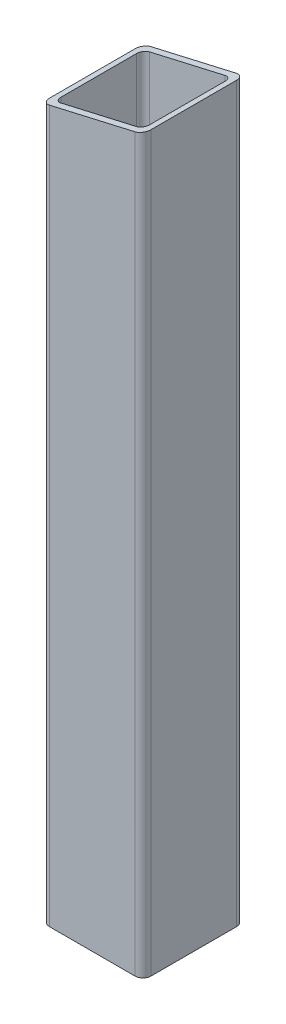
from build123d import *

# Parameters (mm, degrees)
BOSS_EXTRUDE1_DEPTH = 361.5
CUT_EXTRUDE1_REACH  = 390.178


with BuildPart() as part:
    # Sketch2 → Boss-Extrude1 (new, symmetric)
    with BuildSketch(Plane(origin=(0, 0, 0), x_dir=(1, 0, 0), z_dir=(0, 1, 0))):
        with BuildLine():
            Line((7.875, -1.525), (92.125, -1.525))
            ThreePointArc((92.125, -1.525), (97.693465902, 0.781534098), (100, 6.35))
            Line((100, 6.35), (100, 90.6))
            ThreePointArc((100, 90.6), (97.693465902, 96.168465902), (92.125, 98.475))
            Line((92.125, 98.475), (7.875, 98.475))
            ThreePointArc((7.875, 98.475), (2.306534098, 96.168465902), (0, 90.6))
            Line((0, 90.6), (0, 6.35))
            ThreePointArc((0, 6.35), (2.306534098, 0.781534098), (7.875, -1.525))
        make_face()
        with BuildLine():
            Line((12.6, 4.775), (87.4, 4.775))
            ThreePointArc((87.4, 4.775), (91.854772721, 6.620227279), (93.7, 11.075))
            Line((93.7, 11.075), (93.7, 85.875))
            ThreePointArc((93.7, 85.875), (91.854772721, 90.329772721), (87.4, 92.175))
            Line((87.4, 92.175), (12.6, 92.175))
            ThreePointArc((12.6, 92.175), (8.145227279, 90.329772721), (6.3, 85.875))
            Line((6.3, 85.875), (6.3, 11.075))
            ThreePointArc((6.3, 11.075), (8.145227279, 6.620227279), (12.6, 4.775))
        make_face(mode=Mode.SUBTRACT)
    extrude(amount=BOSS_EXTRUDE1_DEPTH, both=True)

    # Sketch4 → Cut-Extrude1 (cut, up to next)
    with BuildSketch(Plane.XY.offset(1.525), mode=Mode.PRIVATE) as cut_extrude1_sk1:
        Polygon((100, 361.5), (0, 338.5), (0, 361.5), align=None)
    cut_extrude1_tool1 = extrude(cut_extrude1_sk1.sketch, amount=-CUT_EXTRUDE1_REACH, mode=Mode.PRIVATE) & part.part
    add(cut_extrude1_tool1.solids().sort_by_distance((33.333333, 353.833333, 1.525))[0], mode=Mode.SUBTRACT)


solid = part.part
